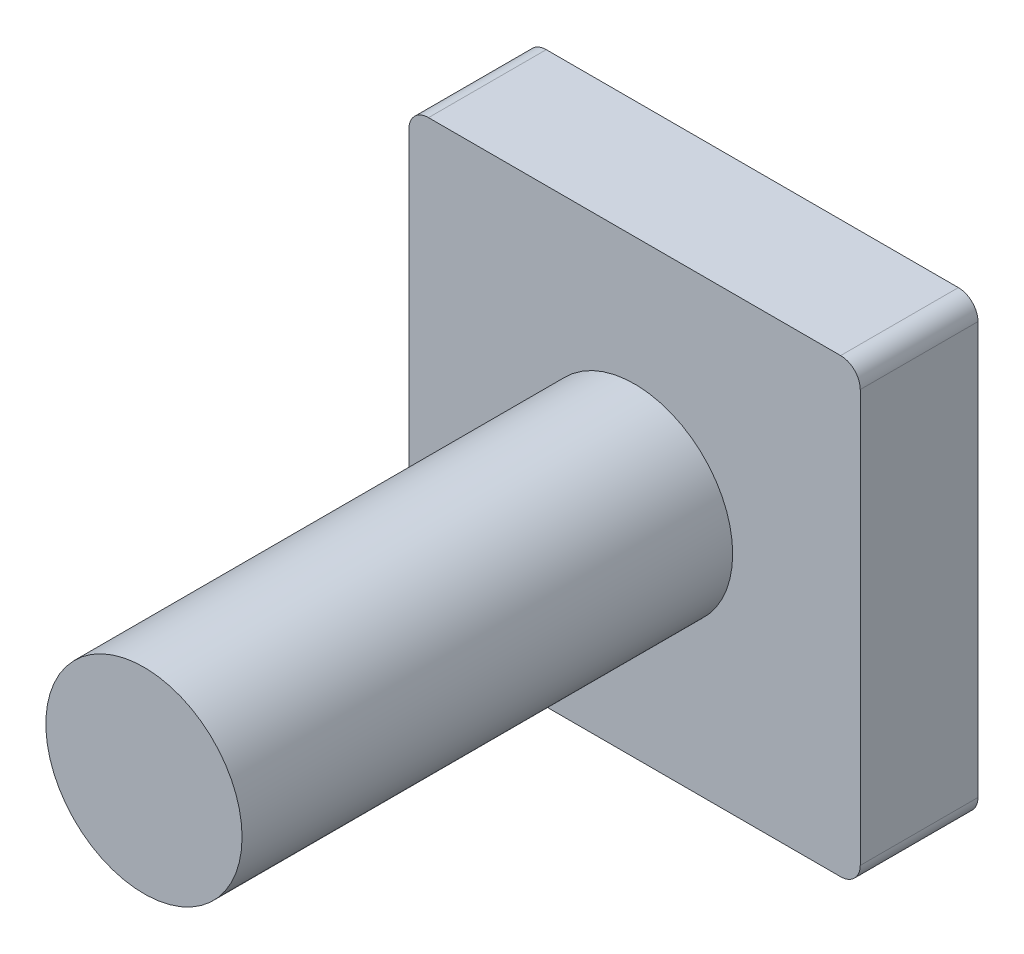
SolidWorks part; units mm, degrees
ref_plane "前视基准面" through (0, 0, 0) normal (0, 0, 1) x (1, 0, 0)
ref_plane "上视基准面" through (0, 0, 0) normal (0, 1, 0) x (1, 0, 0)
ref_plane "右视基准面" through (0, 0, 0) normal (1, 0, 0) x (0, 0, -1)
sketch "草图1" plane through (0, 0, 0) normal (0, 0, 1) x (1, 0, 0)
  circle A0 centre (0, 0) radius 5
  dimension "D1" = 10
extrude "凸台-拉伸1" add sketch "草图1" along normal blind 25
cosmetic thread "装饰螺纹线1" parameters "D2"=9
sketch "草图2" plane through (0, 0, 0) normal (0, 0, -1) x (-1, 0, 0)
  line L1 (11.5, 11.5) -> (-11.5, 11.5)
  line L2 (11.5, 11.5) -> (11.5, -11.5)
  line L3 (11.5, -11.5) -> (-11.5, -11.5)
  line L4 (-11.5, 11.5) -> (-11.5, -11.5)
  line L5 (11.5, 11.5) -> (-11.5, -11.5) construction
  line L6 (11.5, -11.5) -> (-11.5, 11.5) construction
  point P0 (0, 0)
  dimension "D1" = 23
  dimension "D2" = 23
extrude "凸台-拉伸2" add sketch "草图2" along normal blind 6
fillet "圆角1" radius 1 4 edges at (-11.5, 11.5, -3) (-11.5, -11.5, -3) (11.5, 11.5, -3) (11.5, -11.5, -3)
